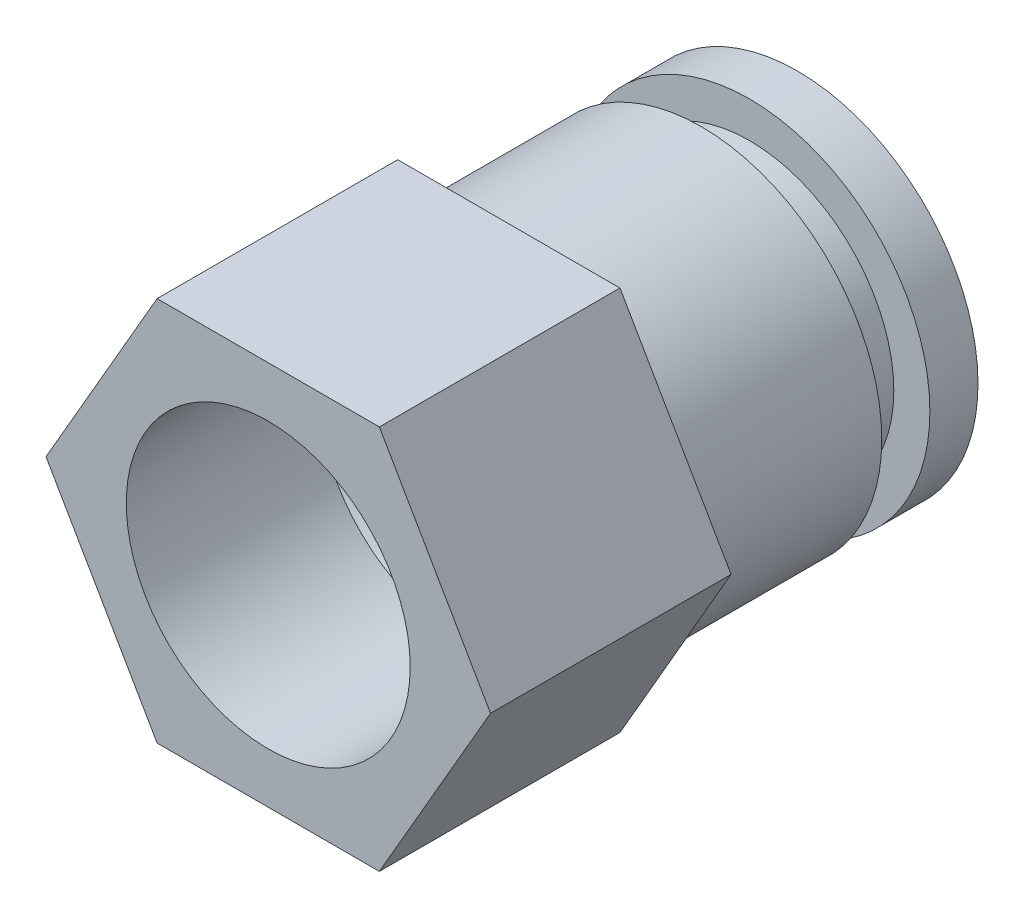
from build123d import *

# Parameters (mm, degrees)
SKETCH1_R               = 7.5
BOSS_EXTRUDE1_DEPTH     = 2
SKETCH2_R               = 6
BOSS_EXTRUDE2_DEPTH     = 2
SKETCH3_R               = 7.5
BOSS_EXTRUDE3_DEPTH     = 8
BOSS_EXTRUDE4_DEPTH     = 10
SKETCH5_R               = 3
CUT_EXTRUDE1_DEPTH      = 26.166114784
G1_4_TAPPED_HOLE1_D     = 11.8
G1_4_TAPPED_HOLE1_DEPTH = 8
G1_4_TAPPED_HOLE1_TIP   = 3.545077652


with BuildPart() as part:
    # Sketch1 → Boss-Extrude1 (new body)
    with BuildSketch(Plane.XY):
        Circle(SKETCH1_R)
    extrude(amount=BOSS_EXTRUDE1_DEPTH)

    # Sketch2 → Boss-Extrude2 (add)
    with BuildSketch(Plane.XY.offset(2)):
        Circle(SKETCH2_R)
    extrude(amount=BOSS_EXTRUDE2_DEPTH)

    # Sketch3 → Boss-Extrude3 (add)
    with BuildSketch(Plane.XY.offset(4)):
        Circle(SKETCH3_R)
    extrude(amount=BOSS_EXTRUDE3_DEPTH)

    # Sketch4 → Boss-Extrude4 (add)
    with BuildSketch(Plane.XY.offset(12)):
        Polygon((9.237604307, 0), (4.618802154, 8), (-4.618802154, 8), (-9.237604307, 0), (-4.618802154, -8), (4.618802154, -8), align=None)
    extrude(amount=BOSS_EXTRUDE4_DEPTH)

    # Sketch5 → Cut-Extrude1 (cut, through all)
    with BuildSketch(Plane(origin=(0, 0, 0), x_dir=(-1, 0, 0), z_dir=(0, 0, -1))):
        Circle(SKETCH5_R)
    extrude(amount=-CUT_EXTRUDE1_DEPTH, mode=Mode.SUBTRACT)

    # G1/4 Tapped Hole1
    with Locations(Plane.XY.offset(22)):
        with Locations((0, 0)):
            Hole(G1_4_TAPPED_HOLE1_D / 2, depth=G1_4_TAPPED_HOLE1_DEPTH)
            with Locations((0, 0, -(G1_4_TAPPED_HOLE1_DEPTH + G1_4_TAPPED_HOLE1_TIP / 2))):  # 118° drill point
                Cone(0, G1_4_TAPPED_HOLE1_D / 2, G1_4_TAPPED_HOLE1_TIP, mode=Mode.SUBTRACT)


solid = part.part
